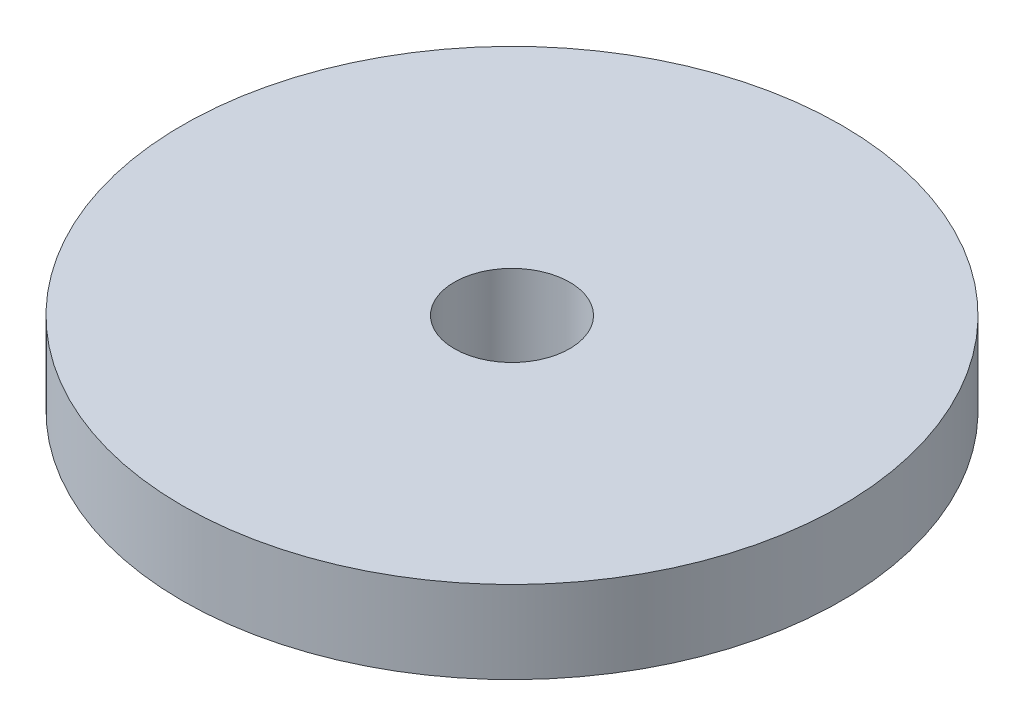
from build123d import *

# Parameters (mm, degrees)
SKETCH_1_R      = 12
SKETCH_1_R_2    = 2.1
EXTRUDE_1_DEPTH = 3


with BuildPart() as part:
    # 草图1 → 凸台-拉伸1 (new body)
    with BuildSketch(Plane(origin=(0, 0, 0), x_dir=(1, 0, 0), z_dir=(0, 1, 0))):
        with Locations(Location((0, 0, 0), (0, 0, 270))):
            Circle(SKETCH_1_R)
        with Locations(Location((0, 0, 0), (0, 0, 270))):
            Circle(SKETCH_1_R_2, mode=Mode.SUBTRACT)
    extrude(amount=EXTRUDE_1_DEPTH)


solid = part.part
